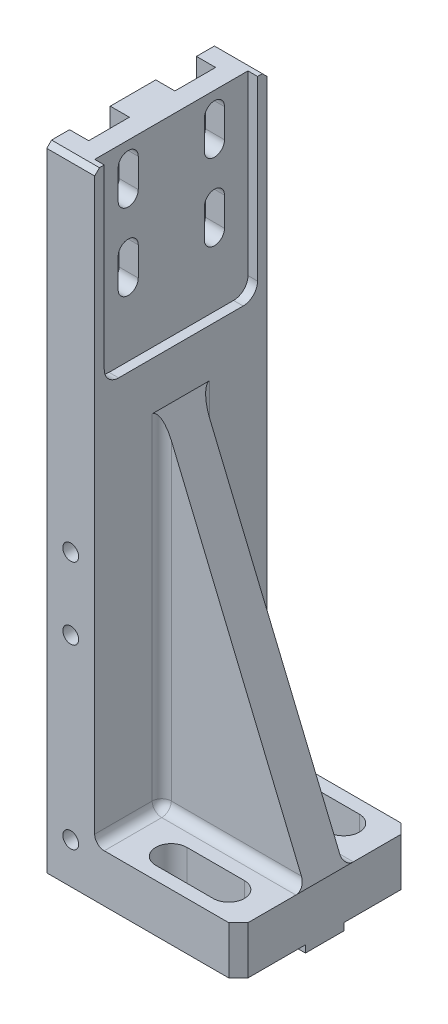
SolidWorks part; units mm, degrees
ref_plane "Front Plane" through (0, 0, 0) normal (0, 0, 1) x (1, 0, 0)
ref_plane "Top Plane" through (0, 0, 0) normal (0, 1, 0) x (1, 0, 0)
ref_plane "Right Plane" through (0, 0, 0) normal (1, 0, 0) x (0, 0, -1)
sketch "Sketch1" plane through (0, 0, 0) normal (0, 0, 1) x (1, 0, 0)
  line L1 (-20, 66) -> (20, 66)
  line L2 (-20, 66) -> (-20, -66)
  line L3 (-20, -66) -> (20, -66)
  line L4 (20, 66) -> (20, -66)
  line L5 (-20, 66) -> (20, -66) construction
  line L6 (-20, -66) -> (20, 66) construction
  point P0 (0, 0)
  dimension "D1" = 40
  dimension "D2" = 132
extrude "Boss-Extrude1" add sketch "Sketch1" along normal mid plane 36
sketch "Sketch2" plane through (0, 0, 18) normal (0, 0, 1) x (1, 0, 0)
  line L0 (-20, 66) -> (-20, -66) construction
  line L1 (20, 66) -> (-10, 66)
  line L2 (20, 66) -> (20, -56)
  line L3 (20, -56) -> (-10, -56)
  line L4 (-10, 66) -> (-10, -56)
  line L5 (-20, -66) -> (20, -66) construction
  dimension "D1" = 10
  dimension "D2" = 10
extrude "Cut-Extrude1" cut sketch "Sketch2" against normal through all
sketch "Sketch3" plane through (0, 0, 0) normal (0, 0, 1) x (1, 0, 0)
  line L0 (20, -56) -> (-10, 16)
  line L1 (-10, 66) -> (-10, -56) construction
  line L2 (-10, 66) -> (-20, 66) construction
  dimension "D1" = 50
rib "Rib2" sketch "Sketch3" sketch "Sketch3" thickness 8 extrusion direction parallel to sketch draft on no parameters "D1"=8
fillet "Fillet1" radius 2 6 edges at (5, -56, -4) (-10, -56, -11) (-10, -20, -4) (5, -56, 4) (-10, -56, 11) (-10, -20, 4)
sketch "Sketch4" plane through (-10, 0, 0) normal (1, 0, 0) x (0, 0, -1)
  line L0 (18, 66) -> (-18, 66) construction
  line L1 (-16, 66) -> (16, 66)
  line L2 (-16, 66) -> (-16, 29)
  line L3 (-13, 26) -> (13, 26)
  line L4 (16, 66) -> (16, 29)
  line L5 (0, 0) -> (0, 79.0395) construction
  line L6 (-18, 66) -> (-18, -54) construction
  arc A0 (16, 29) -> (13, 26) centre (13, 29) cw
  arc A1 (-13, 26) -> (-16, 29) centre (-13, 29) cw
  dimension "D2" = 3
  dimension "D1" = 2
  dimension "D3" = 40
extrude "Cut-Extrude2" cut sketch "Sketch4" against normal blind 2
sketch "Sketch5" plane through (-20, 0, 0) normal (-1, 0, 0) x (0, 0, 1)
  line L0 (-9, 62) -> (-9, 56) construction
  line L1 (-6.9, 62) -> (-6.9, 56)
  line L2 (-11.1, 62) -> (-11.1, 56)
  line L3 (9, 62) -> (9, 56) construction
  line L4 (11.1, 62) -> (11.1, 56)
  line L5 (6.9, 62) -> (6.9, 56)
  line L6 (9, 46) -> (9, 40) construction
  line L7 (11.1, 46) -> (11.1, 40)
  line L8 (6.9, 46) -> (6.9, 40)
  line L9 (-9, 46) -> (-9, 40) construction
  line L10 (-6.9, 46) -> (-6.9, 40)
  line L11 (-11.1, 46) -> (-11.1, 40)
  line L12 (0, 0) -> (0, 62.9246) construction
  line L13 (18, 66) -> (-18, 66) construction
  arc A0 (-6.9, 62) -> (-11.1, 62) centre (-9, 62) ccw
  arc A1 (-11.1, 56) -> (-6.9, 56) centre (-9, 56) ccw
  arc A2 (11.1, 62) -> (6.9, 62) centre (9, 62) ccw
  arc A3 (6.9, 56) -> (11.1, 56) centre (9, 56) ccw
  arc A4 (11.1, 46) -> (6.9, 46) centre (9, 46) ccw
  arc A5 (6.9, 40) -> (11.1, 40) centre (9, 40) ccw
  arc A6 (-6.9, 46) -> (-11.1, 46) centre (-9, 46) ccw
  arc A7 (-11.1, 40) -> (-6.9, 40) centre (-9, 40) ccw
  point P2 (-9, 59)
  point P7 (9, 59)
  point P14 (9, 43)
  point P21 (-9, 43)
  dimension "D1" = 6
  dimension "D2" = 4.2
  dimension "D3" = 18
  dimension "D4" = 7
  dimension "D5" = 16
extrude "Cut-Extrude3" cut sketch "Sketch5" against normal through all
sketch "Sketch8" plane through (-20, 0, 0) normal (-1, 0, 0) x (0, 0, 1)
  line L0 (-9, 56) -> (-9, 66) construction
  line L1 (18, 66) -> (-18, 66) construction
  line L2 (-13.25, 56) -> (-13.25, 66)
  line L3 (-4.75, 56) -> (-4.75, 66)
  line L4 (9, 56) -> (9, 66) construction
  line L5 (4.75, 56) -> (4.75, 66)
  line L6 (13.25, 56) -> (13.25, 66)
  line L7 (-9, 40) -> (-9, 46) construction
  line L8 (-13.25, 40) -> (-13.25, 46)
  line L9 (-4.75, 40) -> (-4.75, 46)
  line L10 (9, 46) -> (9, 40) construction
  line L11 (13.25, 46) -> (13.25, 40)
  line L12 (4.75, 46) -> (4.75, 40)
  arc A0 (-13.25, 56) -> (-4.75, 56) centre (-9, 56) ccw
  arc A1 (-4.75, 66) -> (-13.25, 66) centre (-9, 66) ccw
  arc A2 (4.75, 56) -> (13.25, 56) centre (9, 56) ccw
  arc A3 (13.25, 66) -> (4.75, 66) centre (9, 66) ccw
  arc A4 (-13.25, 40) -> (-4.75, 40) centre (-9, 40) ccw
  arc A5 (-4.75, 46) -> (-13.25, 46) centre (-9, 46) ccw
  arc A6 (13.25, 46) -> (4.75, 46) centre (9, 46) ccw
  arc A7 (4.75, 40) -> (13.25, 40) centre (9, 40) ccw
  point P5 (-9, 61)
  point P10 (9, 61)
  point P18 (-9, 43)
  point P27 (9, 43)
  dimension "D1" = 8.5
  dimension "D2" = 8.5
extrude "Cut-Extrude4" cut sketch "Sketch8" against normal blind 4
sketch "Sketch9" plane through (0, -66, 0) normal (0, -1, 0) x (1, 0, 0)
  line L0 (20, 18) -> (20, -18) construction
  line L1 (-20, 4) -> (20, 4)
  line L2 (-20, 4) -> (-20, -4)
  line L3 (-20, -4) -> (20, -4)
  line L4 (20, 4) -> (20, -4)
  line L5 (-20, 4) -> (20, -4) construction
  line L6 (-20, -4) -> (20, 4) construction
  line L7 (-20, 18) -> (-20, -18) construction
  point P0 (0, 0)
  dimension "D1" = 8
extrude "Boss-Extrude2" add sketch "Sketch9" along normal blind 1.5
sketch "Sketch10" plane through (0, -66, 0) normal (0, -1, 0) x (1, 0, 0)
  line L0 (0, 12) -> (12, 12) construction
  line L1 (0, 15.25) -> (12, 15.25)
  line L2 (0, 8.75) -> (12, 8.75)
  line L3 (0, -12) -> (12, -12) construction
  line L4 (0, -8.75) -> (12, -8.75)
  line L5 (0, -15.25) -> (12, -15.25)
  line L6 (0, 0) -> (25.9922, 0) construction
  line L7 (20, 18) -> (20, 4) construction
  arc A0 (0, 15.25) -> (0, 8.75) centre (0, 12) ccw
  arc A1 (12, 8.75) -> (12, 15.25) centre (12, 12) ccw
  arc A2 (0, -8.75) -> (0, -15.25) centre (0, -12) ccw
  arc A3 (12, -15.25) -> (12, -8.75) centre (12, -12) ccw
  point P2 (6, 12)
  point P7 (6, -12)
  dimension "D1" = 12
  dimension "D2" = 6.5
  dimension "D3" = 24
  dimension "D4" = 8
extrude "Cut-Extrude5" cut sketch "Sketch10" against normal through all
chamfer "Chamfer1" distance 1 angle 45 2 edges at (-15, 66, -18) (-15, 66, 18)
chamfer "Chamfer2" distance 2 angle 45 2 edges at (20, -61, -18) (20, -61, 18)
hole_wizard "M3 Tapped Hole2" positions "Sketch16" profile "Sketch15" tap size "M3" standard "Gb"
sketch "Sketch16" plane through (-20, 0, 0) normal (-1, 0, 0) x (0, 0, 1)
  line L2 (-18, 65) -> (-18, -66) construction
  line L3 (-13.25, 66) -> (-17, 66) construction
  point P0 (-14, 21)
  point P2 (-14, -39)
  dimension "D1" = 4
  dimension "D2" = 60
  dimension "D3" = 45
sketch "Sketch15" plane through (-20, 21, -14) normal (0, 1, 0) x (0, 0, 1)
  line L0 (0, 0) -> (0, 8.2511)
  line L1 (0, 8.2511) -> (1.25, 7.5)
  line L2 (1.25, 7.5) -> (1.25, 0)
  line L5 (1.25, 0) -> (0, 0)
  line L10 (0, 8.2511) -> (-1.25, 7.5) construction
  line L11 (0, -6.35) -> (0, 107.95) construction
  dimension "螺纹孔钻头直径" = 2.5
  dimension "螺纹孔钻头深度" = 7.5
  dimension "导头角度" = 118
cosmetic thread "Hole Thread5" parameters "D1"=6, "D2"=3
cosmetic thread "Hole Thread6" parameters "D1"=6, "D2"=3
hole_wizard "M4 Tapped Hole2" positions "Sketch18" profile "Sketch17" tap size "M4" standard "Gb"
sketch "Sketch18" plane through (0, 0, 18) normal (0, 0, 1) x (1, 0, 0)
  line L0 (-20, 65) -> (-20, -66) construction
  line L3 (-20, 66) -> (-10, 66) construction
  point P0 (-15, -5.5)
  point P2 (-15, -20.5)
  dimension "D1" = 15
  dimension "D2" = 5
  dimension "D3" = 71.5
sketch "Sketch17" plane through (-15, -5.5, 18) normal (1, 0, 0) x (0, -1, 0)
  line L0 (0, 0) -> (0, 12.4914)
  line L1 (0, 12.4914) -> (1.65, 11.5)
  line L2 (1.65, 11.5) -> (1.65, 0)
  line L5 (1.65, 0) -> (0, 0)
  line L10 (0, 12.4914) -> (-1.65, 11.5) construction
  line L11 (0, -6.35) -> (0, 107.95) construction
  dimension "螺纹孔钻头直径" = 3.3
  dimension "螺纹孔钻头深度" = 11.5
  dimension "导头角度" = 118
cosmetic thread "Hole Thread7" parameters "D1"=8, "D2"=4
cosmetic thread "Hole Thread8" parameters "D1"=8, "D2"=4
hole_wizard "M4 Tapped Hole3" positions "Sketch20" profile "Sketch19" tap size "M4" standard "Gb"
sketch "Sketch20" plane through (0, 0, 18) normal (0, 0, 1) x (1, 0, 0)
  line L0 (-20, 65) -> (-20, -66) construction
  line L1 (20, -67.5) -> (-20, -67.5) construction
  point P0 (-15, -57.5)
  dimension "D1" = 5
  dimension "D2" = 10
sketch "Sketch19" plane through (-15, -57.5, 18) normal (1, 0, 0) x (0, -1, 0)
  line L0 (0, 0) -> (0, 12.4914)
  line L1 (0, 12.4914) -> (1.65, 11.5)
  line L2 (1.65, 11.5) -> (1.65, 0)
  line L5 (1.65, 0) -> (0, 0)
  line L10 (0, 12.4914) -> (-1.65, 11.5) construction
  line L11 (0, -6.35) -> (0, 107.95) construction
  dimension "螺纹孔钻头直径" = 3.3
  dimension "螺纹孔钻头深度" = 11.5
  dimension "导头角度" = 118
cosmetic thread "Hole Thread9" parameters "D1"=8, "D2"=4
mirror "Mirror1" about plane through (0, 0, 0) normal (0, 0, 1) of "M4 Tapped Hole3"
